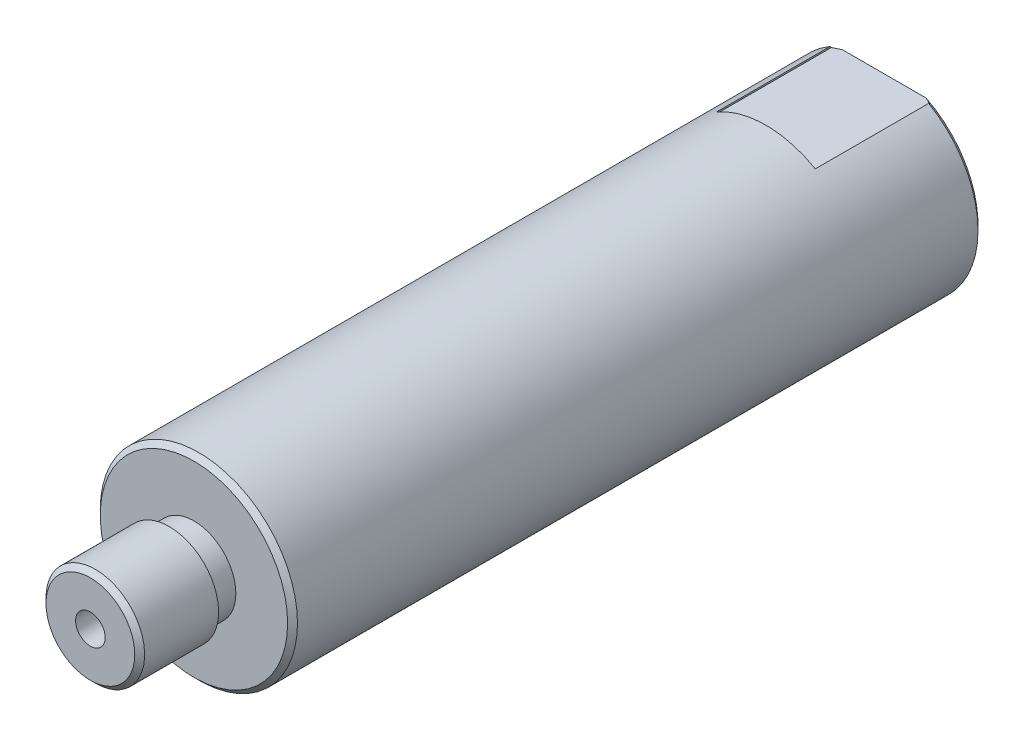
SolidWorks part; units mm, degrees
ref_plane "前视基准面" through (0, 0, 0) normal (0, 0, 1) x (1, 0, 0)
ref_plane "上视基准面" through (0, 0, 0) normal (0, 1, 0) x (1, 0, 0)
ref_plane "右视基准面" through (0, 0, 0) normal (1, 0, 0) x (0, 0, -1)
sketch "草图1" plane through (0, 0, 0) normal (0, 0, 1) x (1, 0, 0)
  circle A0 centre (0, 0) radius 10
  dimension "D1" = 20
extrude "凸台-拉伸1" add sketch "草图1" along normal blind 70
cosmetic thread "装饰螺纹线1" parameters "D2"=18.344
sketch "草图2" plane through (0, 0, 70) normal (0, 0, 1) x (1, 0, 0)
  circle A0 centre (0, 0) radius 5
  dimension "D1" = 10
extrude "凸台-拉伸2" add sketch "草图2" along normal blind 10.5
cosmetic thread "装饰螺纹线2" parameters "D2"=8.891
sketch "草图3" plane through (0, 0, 0) normal (0, 1, 0) x (1, 0, 0)
  line L0 (0, -80.5) -> (0, -63.1949) construction
  line L1 (-5, -70) -> (-4.25, -70)
  line L2 (-5, -70) -> (-5, -72.5)
  line L3 (-5, -72.5) -> (-4.25, -72.5)
  line L4 (-4.25, -70) -> (-4.25, -72.5)
  line L5 (-5, -80.5) -> (5, -80.5) construction
  dimension "D1" = 2.5
  dimension "D2" = 0.75
revolve "切除-旋转1" cut sketch "草图3" angle 360 about L0
sketch "草图4" plane through (0, 0, 80.5) normal (0, 0, 1) x (1, 0, 0)
  circle A0 centre (0, 0) radius 1.5
  dimension "D1" = 3
extrude "切除-拉伸1" cut sketch "草图4" against normal blind 15.5
hole_wizard "1/4 NPT 螺纹孔1" positions "草图6" profile "草图5" size "1/4" standard "ANSI Inch"
sketch "草图6" plane through (0, 0, 0) normal (0, 0, -1) x (-1, 0, 0)
  point P0 (0, 0)
sketch "草图5" plane through (0, 0, 0) normal (1, 0, 0) x (0, 1, 0)
  line L0 (0, 0) -> (0, 20.4123)
  line L1 (5.5626, 17.07) -> (0, 20.4123)
  line L2 (-5.5626, 17.07) -> (0, 20.4123) construction
  line L3 (5.5626, 17.07) -> (5.5626, 10.02)
  line L4 (5.5626, 10.02) -> (5.9437, 10.02)
  line L5 (5.9437, 10.02) -> (6.2437, 0)
  line L6 (-5.9437, 10.02) -> (-6.2437, 0) construction
  line L7 (6.2437, 0) -> (0, 0)
  line L8 (0, -6.35) -> (0, 107.95) construction
  line L11 (-5.5626, 10.02) -> (-5.9437, 10.02) construction
  dimension "螺纹孔钻头直径" = 11.1252
  dimension "螺纹孔钻头深度" = 17.07
  dimension "螺纹直径" = 12.4874
  dimension "螺纹角度" = 3.43
  dimension "螺纹深度" = 10.02
  dimension "导头角度" = 118
cosmetic thread "孔螺蚊线1" parameters "D1"=10.02, "D2"=13.716
hole_wizard "Ø6.0 (6) 直径孔1" positions "草图8" profile "草图7" hole size "Ø6.0" standard "ISO"
sketch "草图8" plane through (0, 0, 65) normal (0, 0, 1) x (1, 0, 0)
  point P0 (0, 0)
sketch "草图7" plane through (0, 0, 65) normal (1, 0, 0) x (0, -1, 0)
  line L0 (0, 0) -> (0, 44.5877)
  line L1 (0, 44.5877) -> (3, 44.5877)
  line L2 (3, 44.5877) -> (3, 0)
  line L5 (3, 0) -> (0, 0)
  line L11 (0, -6.35) -> (0, 107.95) construction
  dimension "通孔孔直径" = 6
  dimension "通孔孔深度" = 44.5877
chamfer "倒角1" distance 0.5 angle 45 3 edges at (10, 0, 0) (10, 0, 70) (5, 0, 80.5)
ref_plane "基准面1" through (0, 10, 0) normal (0, 1, 0) x (1, 0, 0)
sketch "草图9" plane through (0, 10, 0) normal (0, 1, 0) x (1, 0, 0)
  line L0 (9.5, 0) -> (-9.5, 0) construction
  line L1 (-5, 0) -> (5, 0)
  line L2 (-5, 0) -> (-5, -12)
  line L3 (-5, -12) -> (5, -12)
  line L4 (5, 0) -> (5, -12)
  dimension "D1" = 12
  dimension "D2" = 10
  dimension "D3" = 5
extrude "切除-拉伸2" cut sketch "草图9" against normal blind 1.5
mirror "镜向1" about plane through (0, 0, 0) normal (0, 1, 0) of "切除-拉伸2"
